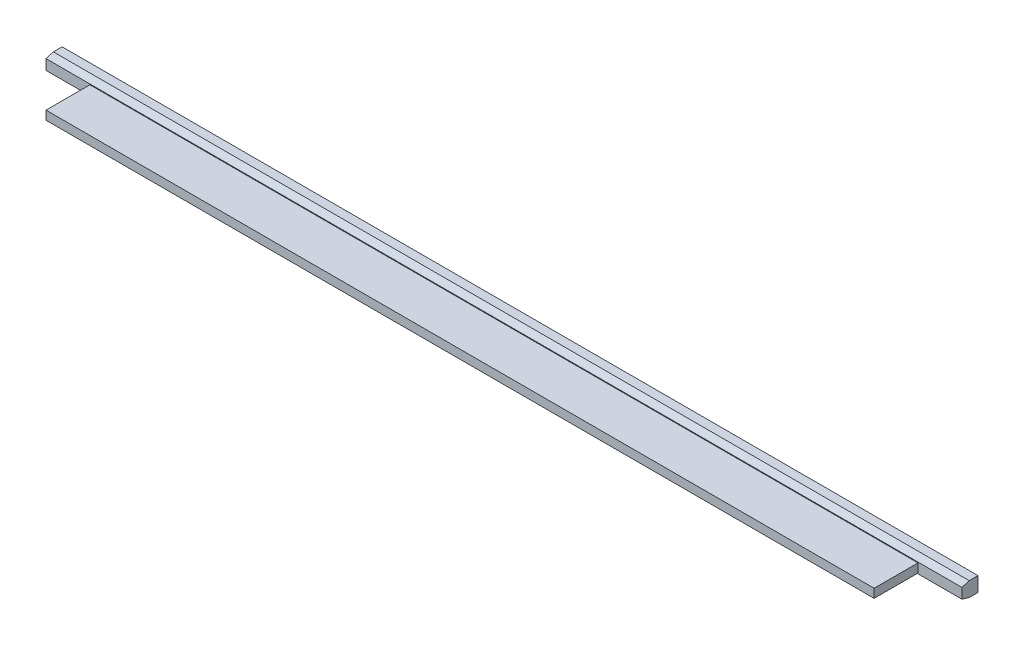
SolidWorks part; units mm, degrees
ref_plane "Front Plane" through (0, 0, 0) normal (0, 0, 1) x (1, 0, 0)
ref_plane "Top Plane" through (0, 0, 0) normal (0, 1, 0) x (1, 0, 0)
ref_plane "Right Plane" through (0, 0, 0) normal (1, 0, 0) x (0, 0, -1)
sketch "Sketch1" plane through (0, 0, 0) normal (0, 0, 1) x (1, 0, 0)
  line L1 (-156.5, 2.5) -> (156.5, 2.5)
  line L2 (-156.5, 2.5) -> (-156.5, -2.5)
  line L3 (-156.5, -2.5) -> (156.5, -2.5)
  line L4 (156.5, 2.5) -> (156.5, -2.5)
  line L5 (-156.5, 2.5) -> (156.5, -2.5) construction
  line L6 (-156.5, -2.5) -> (156.5, 2.5) construction
  point P0 (0, 0)
  dimension "D1" = 5
  dimension "D2" = 313
extrude "Boss-Extrude1" add sketch "Sketch1" along normal blind 5.5
sketch "Sketch3" plane through (156.5, 0, 0) normal (1, 0, 0) x (0, 0, -1)
  line L0 (-3, 2.5) -> (-5.5, 1.75)
  line L1 (-5.5, 2.5) -> (0, 2.5) construction
  line L2 (-5.5, -2.5) -> (-5.5, 2.5) construction
  line L3 (-3, -2.5) -> (-5.5, -1.75)
  line L4 (-5.5, -2.5) -> (0, -2.5) construction
  line L5 (0, 0) -> (-1.9318, 0) construction
  line L6 (0, -2.5) -> (0, 2.5) construction
  line L7 (-5.5, 1.75) -> (-5.5, 2.5)
  line L8 (-5.5, 2.5) -> (-3, 2.5)
  line L9 (-5.5, -1.75) -> (-5.5, -2.5)
  line L10 (-5.5, -2.5) -> (-3, -2.5)
  dimension "D1" = 3
  dimension "D2" = 3.5
extrude "Cut-Extrude1" cut sketch "Sketch3" against normal through all
sketch "Sketch2" plane through (0, 0, 5.5) normal (0, 0, 1) x (1, 0, 0)
  line L1 (156.5, -1.75) -> (156.5, 1.75) construction
  line L2 (-141.5, -1.5) -> (141.5, -1.5)
  line L3 (-141.5, -1.5) -> (-141.5, 1.5)
  line L4 (-141.5, 1.5) -> (141.5, 1.5)
  line L5 (141.5, -1.5) -> (141.5, 1.5)
  line L6 (-141.5, -1.5) -> (141.5, 1.5) construction
  line L7 (-141.5, 1.5) -> (141.5, -1.5) construction
  point P0 (0, 0)
  dimension "D1" = 3
  dimension "D2" = 15
extrude "Boss-Extrude2" add sketch "Sketch2" along normal blind 15
